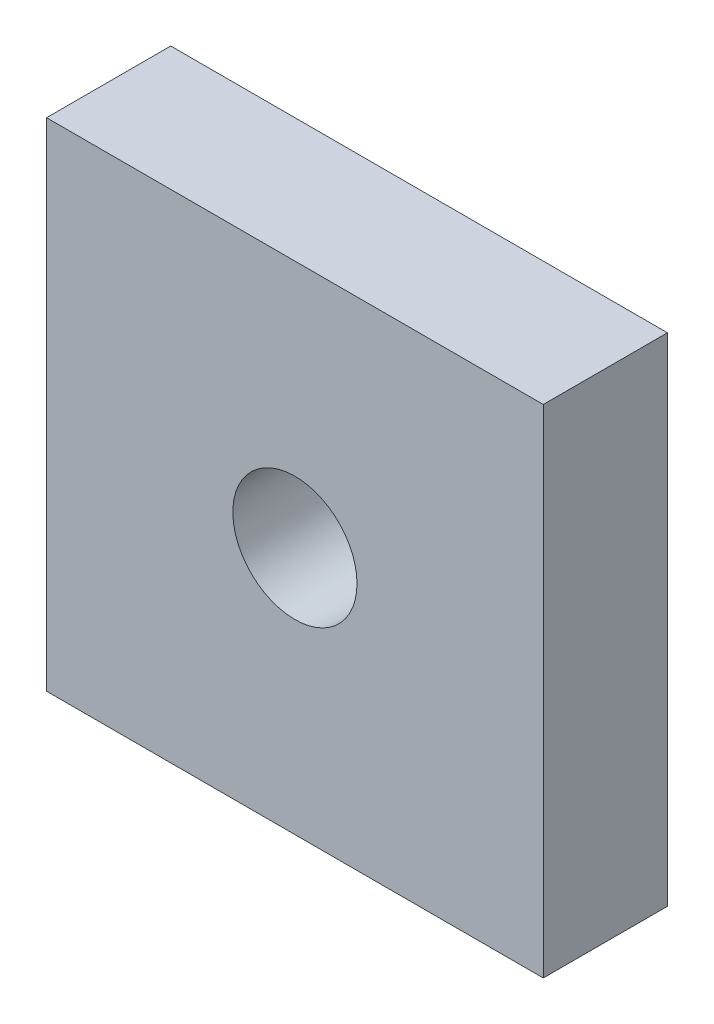
SolidWorks part; units mm, degrees
material "Q235B"
ref_plane "Front Plane" through (0, 0, 0) normal (0, 0, 1) x (1, 0, 0)
ref_plane "Top Plane" through (0, 0, 0) normal (0, 1, 0) x (1, 0, 0)
ref_plane "Right Plane" through (0, 0, 0) normal (1, 0, 0) x (0, 0, -1)
sketch "Sketch1" plane through (0, 0, 0) normal (0, 0, 1) x (1, 0, 0)
  line L1 (0, 0) -> (40, 0)
  line L2 (0, 0) -> (0, 40)
  line L3 (0, 40) -> (40, 40)
  line L4 (40, 0) -> (40, 40)
  circle A0 centre (20, 20) radius 5
  dimension "D3" = 10
  dimension "D4" = 20
  dimension "D5" = 20
  dimension "D1" = 40
  dimension "D2" = 40
extrude "Boss-Extrude1" add sketch "Sketch1" along normal blind 10
